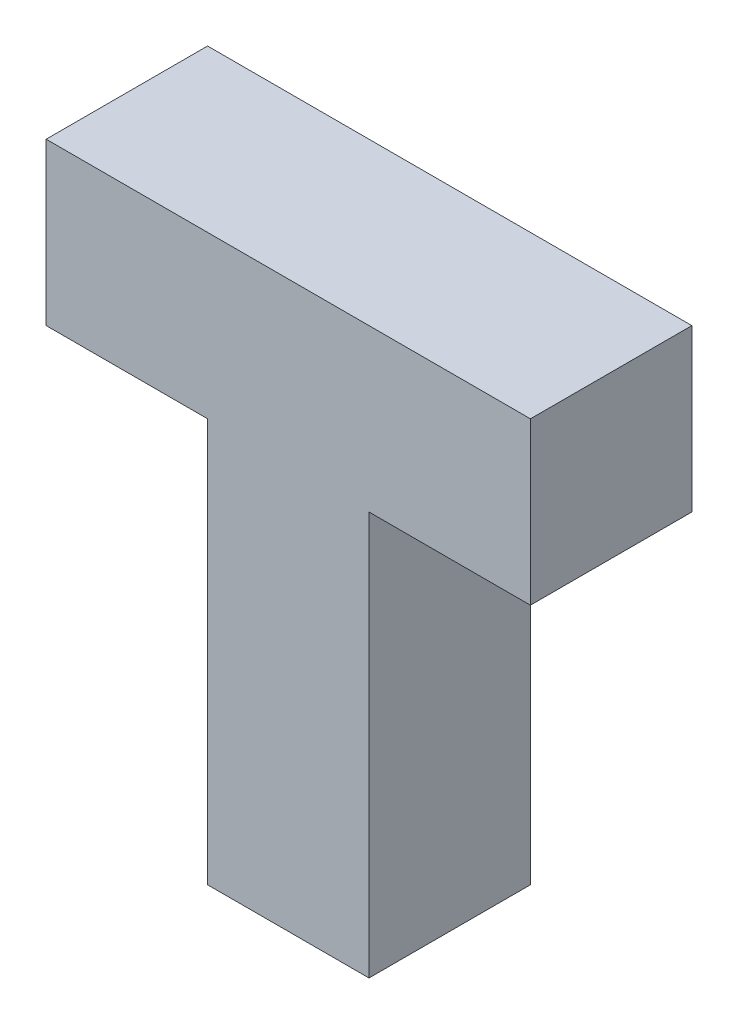
from build123d import *

# Parameters (mm, degrees)
SKETCH1_W           = 30
SKETCH1_H           = 35
BOSS_EXTRUDE1_DEPTH = 10
SKETCH2_W           = 10
SKETCH2_H           = 25
CUT_EXTRUDE1_DEPTH  = 26.124689053


with BuildPart() as part:
    # Sketch1 → Boss-Extrude1 (new body)
    with BuildSketch(Plane.XY):
        Rectangle(SKETCH1_W, SKETCH1_H)
    extrude(amount=BOSS_EXTRUDE1_DEPTH)

    # Sketch2 → Cut-Extrude1 (cut, through all)
    with BuildSketch(Plane.XY.offset(10)):
        with Locations((-10, -5)):
            Rectangle(SKETCH2_W, SKETCH2_H)
        with Locations((10, -5)):
            Rectangle(SKETCH2_W, SKETCH2_H)
    extrude(amount=-CUT_EXTRUDE1_DEPTH, mode=Mode.SUBTRACT)


solid = part.part
